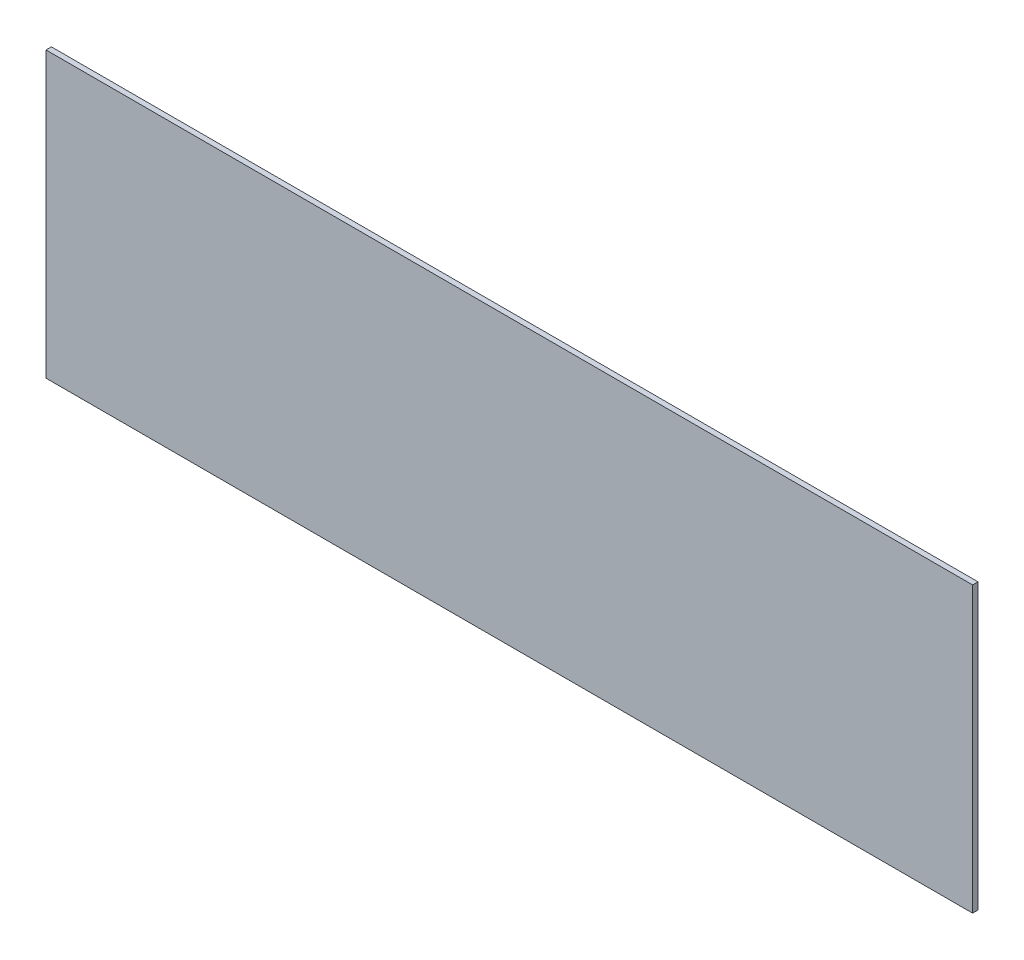
from build123d import *

# Parameters (mm, degrees)
SKETCH1_W           = 515
SKETCH1_H           = 158
BOSS_EXTRUDE1_DEPTH = 3


with BuildPart() as part:
    # Sketch1 → Boss-Extrude1 (new body)
    with BuildSketch(Plane.XY):
        Rectangle(SKETCH1_W, SKETCH1_H)
    extrude(amount=BOSS_EXTRUDE1_DEPTH)


solid = part.part
